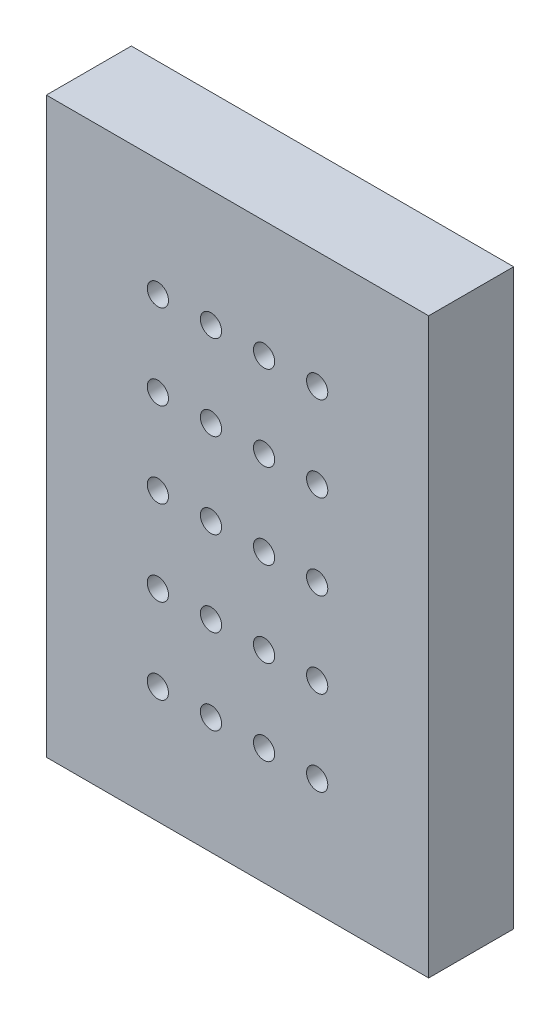
SolidWorks part; units mm, degrees
ref_plane "前视基准面" through (0, 0, 0) normal (0, 0, 1) x (1, 0, 0)
ref_plane "上视基准面" through (0, 0, 0) normal (0, 1, 0) x (1, 0, 0)
ref_plane "右视基准面" through (0, 0, 0) normal (1, 0, 0) x (0, 0, -1)
sketch "草图1" plane through (0, 0, 0) normal (0, 0, 1) x (1, 0, 0)
  line L1 (-9, -13.5) -> (9, -13.5)
  line L2 (-9, -13.5) -> (-9, 13.5)
  line L3 (-9, 13.5) -> (9, 13.5)
  line L4 (9, -13.5) -> (9, 13.5)
  line L5 (-9, -13.5) -> (9, 13.5) construction
  line L6 (-9, 13.5) -> (9, -13.5) construction
  point P0 (0, 0)
  dimension "D1" = 18
  dimension "D2" = 27
extrude "凸台-拉伸1" add sketch "草图1" along normal blind 4
sketch "草图2" plane through (0, 0, 4) normal (0, 0, 1) x (1, 0, 0)
  circle A0 centre (-1.25, 0) radius 0.5
  circle A1 centre (-3.75, 0) radius 0.5
  circle A2 centre (1.25, 0) radius 0.5
  circle A3 centre (3.75, 0) radius 0.5
extrude "切除-拉伸1" cut sketch "草图2" against normal up to next
pattern_linear "阵列(线性)2" count 3 spacing 4 along (0, -1, 0) of "切除-拉伸1"
mirror "镜向1" about plane through (0, 0, 0) normal (0, 1, 0) of "阵列(线性)2"
sketch "草图3" plane through (0, 0, 0) normal (0, 0, -1) x (-1, 0, 0)
  line L0 (9, 13.5) -> (9, -13.5) construction
  line L1 (-5.8, 12.3) -> (5.8, 12.3)
  line L2 (-7.8, 10.3) -> (-7.8, -10.3)
  line L3 (-5.8, -12.3) -> (5.8, -12.3)
  line L4 (7.8, 10.3) -> (7.8, -10.3)
  line L5 (-7.8, 12.3) -> (7.8, -12.3) construction
  line L6 (-7.8, -12.3) -> (7.8, 12.3) construction
  line L7 (-9, 13.5) -> (9, 13.5) construction
  arc A0 (-7.8, -10.3) -> (-5.8, -12.3) centre (-5.8, -10.3) ccw
  arc A1 (5.8, -12.3) -> (7.8, -10.3) centre (5.8, -10.3) ccw
  arc A2 (-5.8, 12.3) -> (-7.8, 10.3) centre (-5.8, 10.3) ccw
  arc A3 (5.8, 12.3) -> (7.8, 10.3) centre (5.8, 10.3) cw
  point P0 (0, 0)
equation "\"D3@草图2\"=\"D2@草图2\""
equation "\"D3@草图3\"=\"D2@草图3\""
equation "\"D5@草图2\"=\"D2@草图2\""
